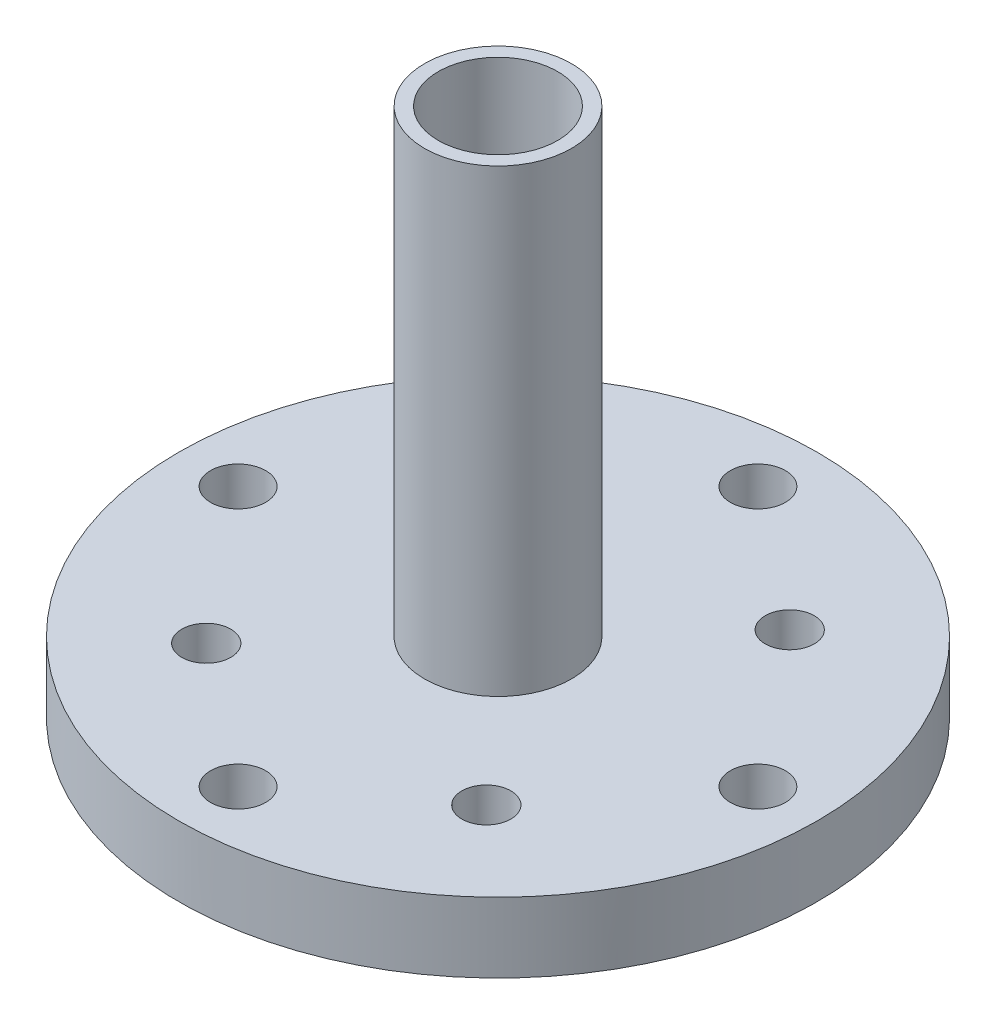
from build123d import *

# Parameters (mm, degrees)
SKETCH1_R           = 31.75
SKETCH1_R_2         = 2.667
BOSS_EXTRUDE1_DEPTH = 7.62
SKETCH2_R           = 6.604
CUT_EXTRUDE1_DEPTH  = 46.543269536
SKETCH_1_R          = 7.5
EXTRUDE_1_DEPTH     = 7.62
SKETCH_2_R          = 8
SKETCH_2_R_2        = 6.5
BOSS_EXTRUDE2_DEPTH = 50
SCALE1_SCALE        = 2
SKETCH3_R           = 6
CUT_EXTRUDE_1_DEPTH = 21
BOSS_EXTRUDE3_START = -15.24
SKETCH5_R           = 69.5
SKETCH5_R_2         = 63.5
BOSS_EXTRUDE3_DEPTH = 15.24


with BuildPart() as part:
    # Sketch1 → Boss-Extrude1 (new body)
    with BuildSketch(Plane(origin=(0, 0, 0), x_dir=(1, 0, 0), z_dir=(0, 1, 0))):
        with Locations(Location((0, 0, 0), (0, 0, 270))):
            Circle(SKETCH1_R)
        with Locations(Location((-15.24, 16.51, 0), (0, 0, 270))):
            Circle(SKETCH1_R_2, mode=Mode.SUBTRACT)
        with Locations(Location((15.24, 16.51, 0), (0, 0, 270))):
            Circle(SKETCH1_R_2, mode=Mode.SUBTRACT)
        with Locations(Location((15.24, -16.51, 0), (0, 0, 270))):
            Circle(SKETCH1_R_2, mode=Mode.SUBTRACT)
        with Locations(Location((-15.24, -16.51, 0), (0, 0, 270))):
            Circle(SKETCH1_R_2, mode=Mode.SUBTRACT)
    extrude(amount=-BOSS_EXTRUDE1_DEPTH)

    # Sketch2 → Cut-Extrude1 (cut, through all)
    with BuildSketch(Plane(origin=(0, 0, 0), x_dir=(1, 0, 0), z_dir=(0, 1, 0))):
        with Locations(Location((0, 0, 0), (0, 0, 270))):
            Circle(SKETCH2_R)
    extrude(amount=-CUT_EXTRUDE1_DEPTH, mode=Mode.SUBTRACT)

    # 草图1 → 凸台-拉伸1 (add)
    with BuildSketch(Plane.XZ.offset(7.62)):
        Circle(SKETCH_1_R)
    extrude(amount=-EXTRUDE_1_DEPTH)

    # 草图2 → Boss-Extrude2 (add)
    with BuildSketch(Plane(origin=(0, 0, 0), x_dir=(1, 0, 0), z_dir=(0, 1, 0))):
        with Locations(Location((0, 0, 0), (0, 0, 270))):
            Circle(SKETCH_2_R)
        with Locations(Location((0, 0, 0), (0, 0, 270))):
            Circle(SKETCH_2_R_2, mode=Mode.SUBTRACT)
    extrude(amount=BOSS_EXTRUDE2_DEPTH)


with BuildPart() as part_1:
    # Scale1: scaled about (0, 0, 0)
    add(part.part.scale(SCALE1_SCALE))

    # Sketch3 → 切除-拉伸1 (cut)
    with BuildSketch(Plane(origin=(0, 0, 0), x_dir=(1, 0, 0), z_dir=(0, 1, 0))):
        with Locations(Location((56.568542495, 0, 0), (0, 0, 270))):
            Circle(SKETCH3_R)
        with Locations(Location((0, -56.568542495, 0), (0, 0, 270))):
            Circle(SKETCH3_R)
        with Locations(Location((-56.568542495, 0, 0), (0, 0, 270))):
            Circle(SKETCH3_R)
        with Locations(Location((0, 56.568542495, 0), (0, 0, 270))):
            Circle(SKETCH3_R)
    extrude(amount=-CUT_EXTRUDE_1_DEPTH, mode=Mode.SUBTRACT)

    # Sketch5 → Boss-Extrude3 (add)
    with BuildSketch(Plane.XZ.offset(15.24).offset(BOSS_EXTRUDE3_START)):
        with Locations(Location((0, 0, 0), (0, 0, 270))):
            Circle(SKETCH5_R)
        Circle(SKETCH5_R_2, mode=Mode.SUBTRACT)
    extrude(amount=BOSS_EXTRUDE3_DEPTH)


solid = part_1.part
